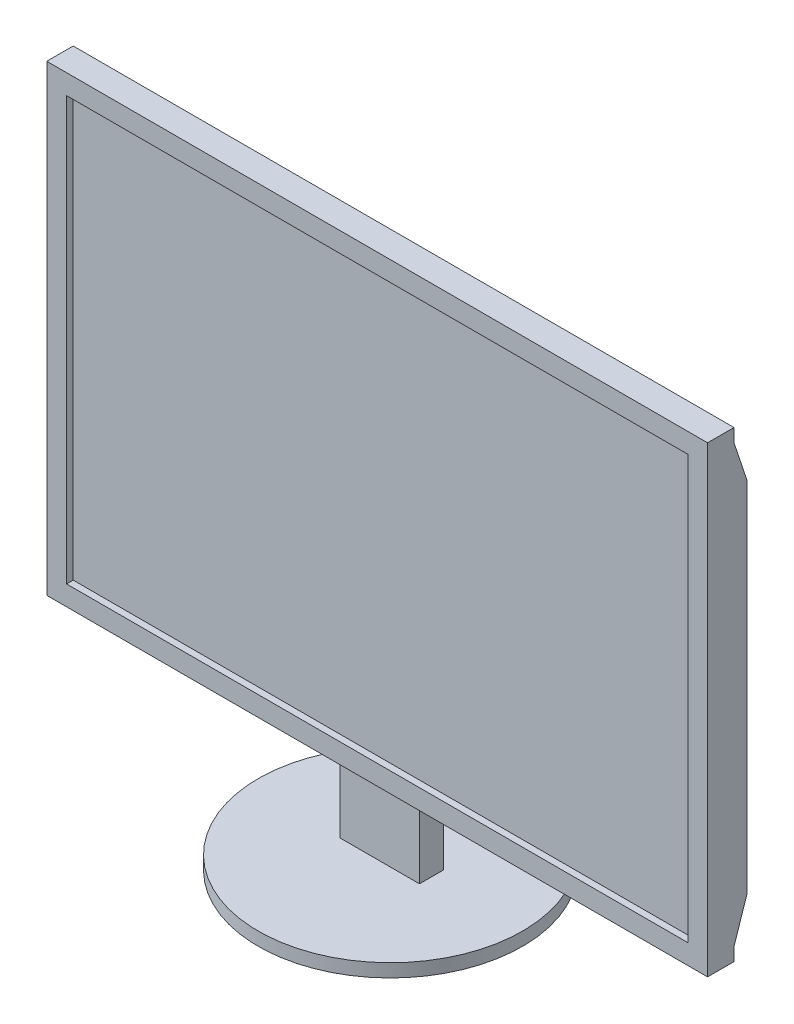
from build123d import *

# Parameters (mm, degrees)
SKETCH1_W           = 500
SKETCH1_H           = 350
BOSS_EXTRUDE1_DEPTH = 20
BOSS_EXTRUDE2_DEPTH = 500
SKETCH3_W           = 470
SKETCH3_H           = 320
CUT_EXTRUDE1_DEPTH  = 5
SKETCH4_W           = 60
SKETCH4_H           = 18
BOSS_EXTRUDE3_DEPTH = 50
SKETCH5_R           = 100
BOSS_EXTRUDE4_DEPTH = 10


with BuildPart() as part:
    # Sketch1 → Boss-Extrude1 (new body)
    with BuildSketch(Plane.XY):
        with Locations((250, 175)):
            Rectangle(SKETCH1_W, SKETCH1_H)
    extrude(amount=BOSS_EXTRUDE1_DEPTH)

    # Sketch2 → Boss-Extrude2 (add)
    with BuildSketch(Plane(origin=(500, 0, 0), x_dir=(0, 0, -1), z_dir=(1, 0, 0))):
        Polygon((0, 340), (0, 10), (10, 40), (10, 310), align=None)
    extrude(amount=-BOSS_EXTRUDE2_DEPTH)

    # Sketch3 → Cut-Extrude1 (cut)
    with BuildSketch(Plane.XY.offset(20)):
        with Locations((250, 175)):
            Rectangle(SKETCH3_W, SKETCH3_H)
    extrude(amount=-CUT_EXTRUDE1_DEPTH, mode=Mode.SUBTRACT)

    # Sketch4 → Boss-Extrude3 (add)
    with BuildSketch(Plane.XZ):
        with Locations((250, 9)):
            Rectangle(SKETCH4_W, SKETCH4_H)
    extrude(amount=BOSS_EXTRUDE3_DEPTH)

    # Sketch5 → Boss-Extrude4 (add)
    with BuildSketch(Plane.XZ.offset(50)):
        with Locations(Location((250, 10, 0), (0, 0, 270))):
            Circle(SKETCH5_R)
    extrude(amount=BOSS_EXTRUDE4_DEPTH)


solid = part.part
